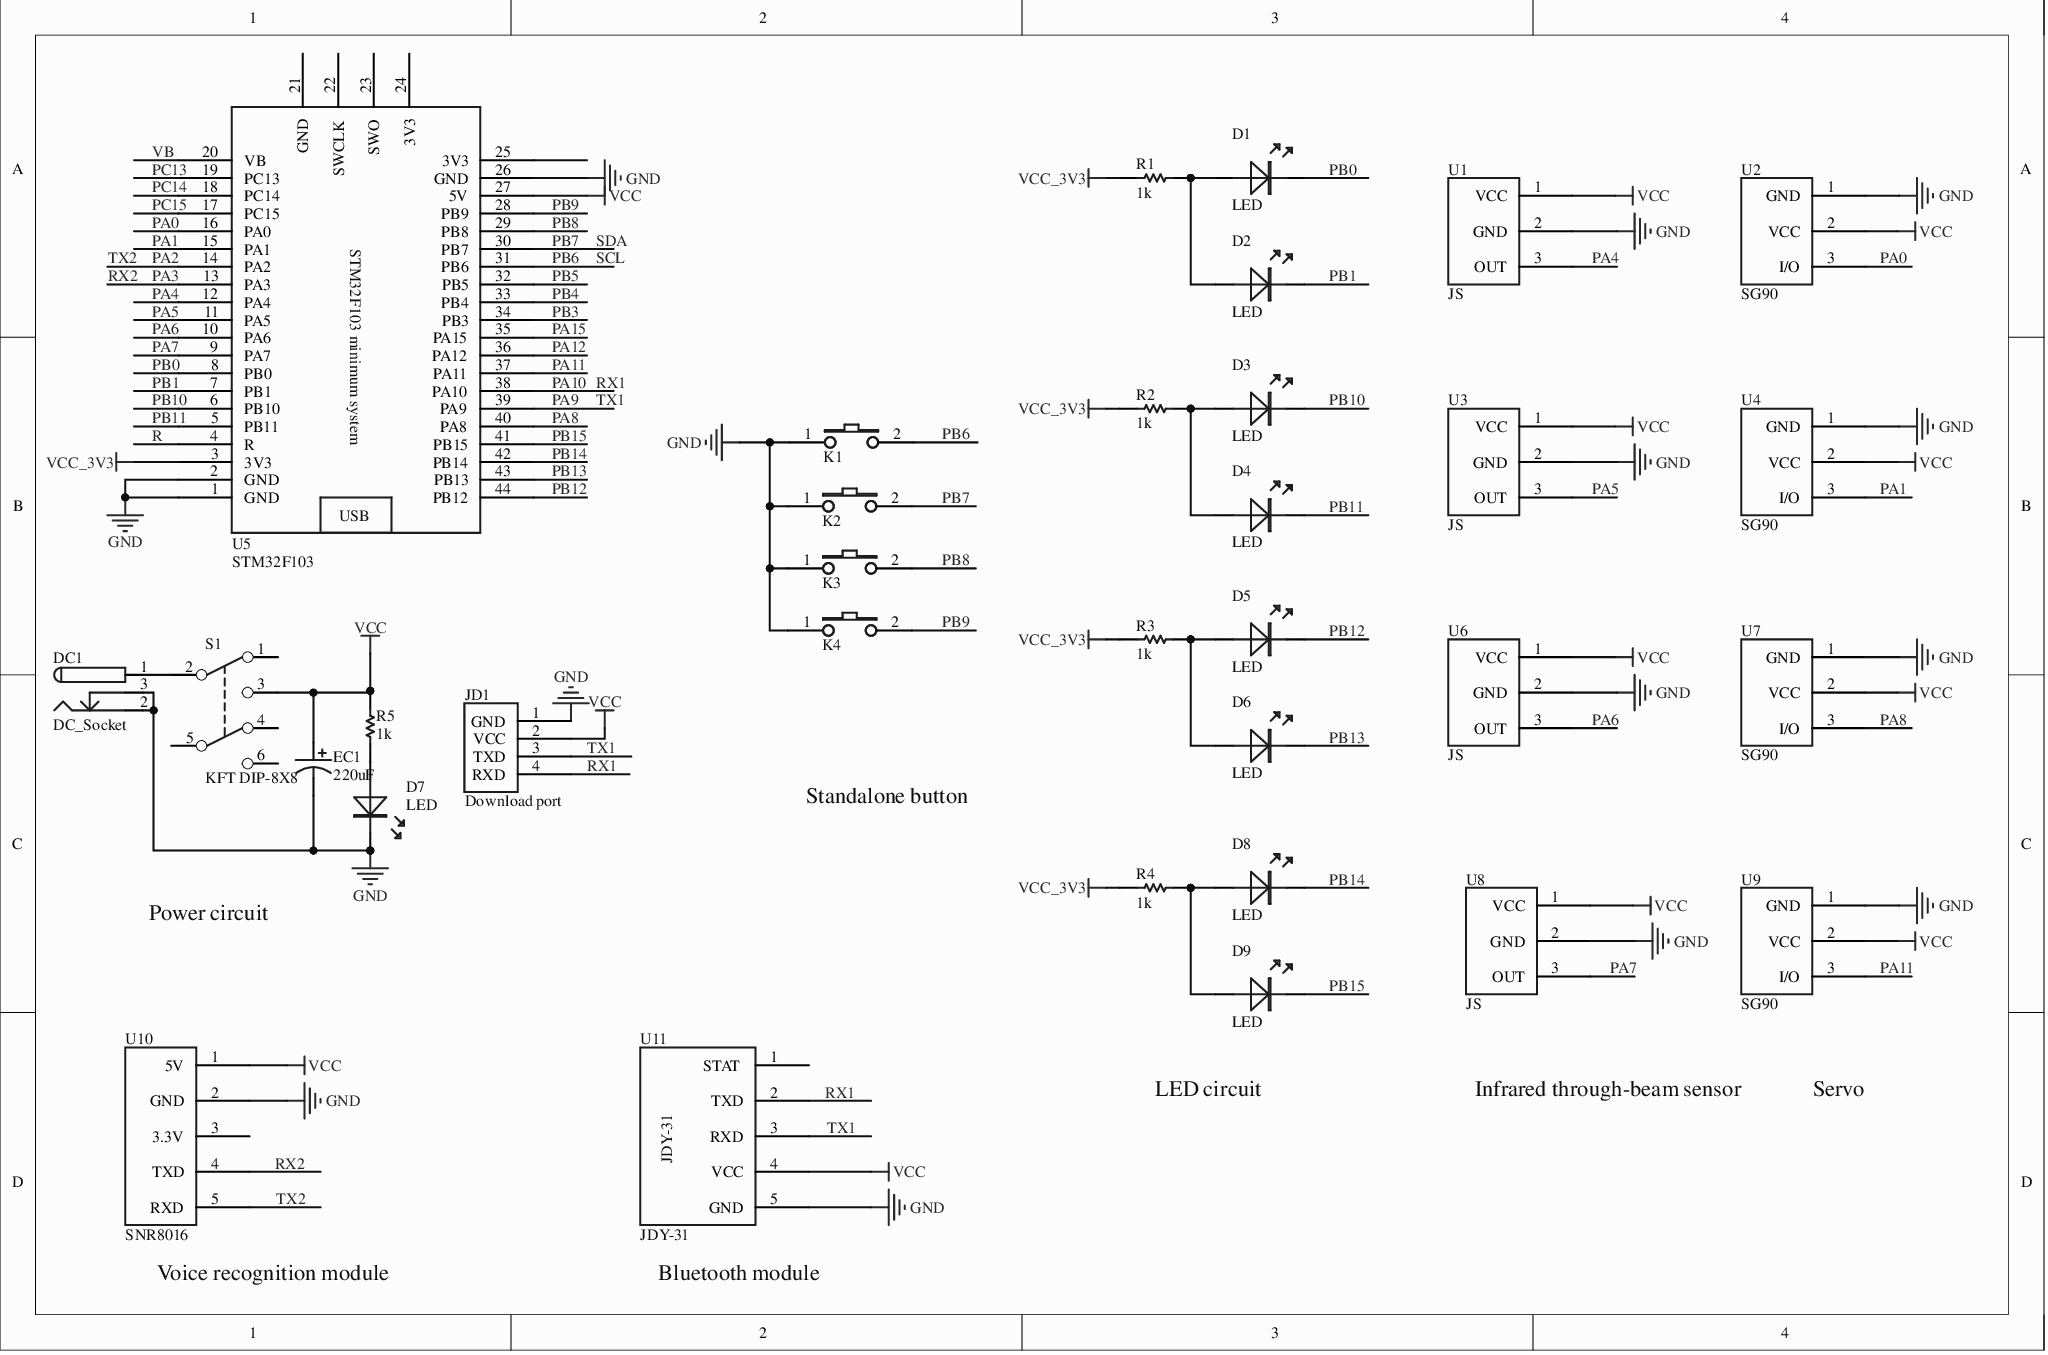
[diagram p0: MISC49929-2.schdoc]
# Altium project MISC49929.PrjPcb
1 sheet, 33 parts. Net scope: global (net labels, ports and power ports of the same name join across sheets).
Board file: MISC49929.pcbdoc

## Sheet MISC49929-2.schdoc
size 292 x 193 mm; Name: MISC49929

### Parts
D1  LED  [LED5-GRE]
D2  LED  [LED5-RED]
D3  LED  [LED5-GRE]
D4  LED  [LED5-RED]
D5  LED  [LED5-GRE]
D6  LED  [LED5-RED]
D7  LED  [LED5-GRE]
D8  LED  [LED5-GRE]
D9  LED  [LED5-RED]
DC1  DC_Socket  [DC-005]
EC1  220uF  [DIP-EC3.5X8X11.5]
JD1  Download port  [下载口]
K1  BUTTOM  [DIP-6X6X5]  (value not drawn)
K2  BUTTOM  [DIP-6X6X5]  (value not drawn)
K3  BUTTOM  [DIP-6X6X5]  (value not drawn)
K4  BUTTOM  [DIP-6X6X5]  (value not drawn)
R1  1k  [AXIAL0.3-1k]
R2  1k  [AXIAL0.3-1k]
R3  1k  [AXIAL0.3-1k]
R4  1k  [AXIAL0.3-1k]
R5  1k  [AXIAL0.3-1k]
S1  KFT DIP-8X8  [KFT DIP-8X8]
U1  JS  [JS]
U2  SG90  [SG90]
U3  JS  [JS]
U4  SG90  [SG90]
U5  STM32F103  [STM32F103]
U6  JS  [JS]
U7  SG90  [SG90]
U8  JS  [JS]
U9  SG90  [SG90]
U10  SNR8016  [SNR8016]
U11  JDY-31

### Nets
GND: D7.K DC1.2 DC1.3 EC1.2 JD1.1(GND) K1.1 K2.1 K3.1 K4.1 U1.2(GND) U2.1(GND) U3.2(GND) U4.1(GND) U5.1(GND) U5.2(GND) U5.26(GND) U6.2(GND) U7.1(GND) U8.2(GND) U9.1(GND) U10.2(GND) U11.5(GND)
VCC: EC1.1 JD1.2(VCC) R5.2 S1.3 U1.1(VCC) U2.2(VCC) U3.1(VCC) U4.2(VCC) U5.27(5V) U6.1(VCC) U7.2(VCC) U8.1(VCC) U9.2(VCC) U10.1(5V) U11.4(VCC)
VCC_3V3: R1.2 R2.2 R3.2 R4.2 U5.3(3V3)
PA0: U2.3(I/O) U5.16(PA0)
PA1: U4.3(I/O) U5.15(PA1)
PA2: U5.14(PA2) U10.5(RXD)  [also labelled TX2]
PA3: U5.13(PA3) U10.4(TXD)  [also labelled RX2]
PA4: U1.3(OUT) U5.12(PA4)
PA5: U3.3(OUT) U5.11(PA5)
PA6: U5.10(PA6) U6.3(OUT)
PA7: U5.9(PA7) U8.3(OUT)
PA8: U5.40(PA8) U7.3(I/O)
PA9: JD1.3(TXD) U5.39(PA9) U11.3(RXD)  [also labelled TX1]
PA10: JD1.4(RXD) U5.38(PA10) U11.2(TXD)  [also labelled RX1]
PA11: U5.37(PA11) U9.3(I/O)
PA12: U5.36(PA12)
PA15: U5.35(PA15)
PB0: D1.K U5.8(PB0)
PB1: D2.K U5.7(PB1)
PB3: U5.34(PB3)
PB4: U5.33(PB4)
PB5: U5.32(PB5)
PB6: K1.2 U5.31(PB6)  [also labelled SCL]
PB7: K2.2 U5.30(PB7)  [also labelled SDA]
PB8: K3.2 U5.29(PB8)
PB9: K4.2 U5.28(PB9)
PB10: D3.K U5.6(PB10)
PB11: D4.K U5.5(PB11)
PB12: D5.K U5.44(PB12)
PB13: D6.K U5.43(PB13)
PB14: D8.K U5.42(PB14)
PB15: D9.K U5.41(PB15)
PC13: U5.19(PC13)
PC14: U5.18(PC14)
PC15: U5.17(PC15)
R: U5.4(R)
VB: U5.20(VB)
NetD1_A: D1.A D2.A R1.1
NetD3_A: D3.A D4.A R2.1
NetD5_A: D5.A D6.A R3.1
NetD7_A: D7.A R5.1
NetD8_A: D8.A D9.A R4.1
NetDC1_1: DC1.1 S1.2

Not connected (* = marked no-connect by the designer): S1 1 4 5 6; U5 21(GND) 22(SWCLK) 23(SWO) 24(3V3) 25(3V3); U10 3(3.3V)*; U11 1(STAT)*

### Notes on the sheet
- Standalone button
- Power circuit
- LED circuit
- Infrared through-beam sensor
- Servo
- (near U10) Voice recognition module
- (near U11) Bluetooth module

### Library data of the parts
D1 = LED: LED red; Origin Footprint: LED5-BLUE; OriginFootprint 3: LED5-YEL; UniqueId: 07a0d5848cd81316; AddInBom: yes; Device: LED; OriginFootprint 2: LED5-GRE; DesignItemID: LED; LibraryName: LED; SymbolName: LED; FootprintName: LED5-GRE
D2 = LED_1: LED red; Origin Footprint: LED5-BLUE; OriginFootprint 2: LED5-GRE; OriginFootprint 3: LED5-YEL; UniqueId: fa5cd661465da5bc; AddInBom: yes; Device: LED_1; DesignItemID: LED; LibraryName: LED; SymbolName: LED; FootprintName: LED5-RED
D3 = LED: LED red; Origin Footprint: LED5-BLUE; OriginFootprint 3: LED5-YEL; UniqueId: ce0e29427420bb9a; AddInBom: yes; Device: LED; OriginFootprint 2: LED5-GRE; DesignItemID: LED; LibraryName: LED; SymbolName: LED; FootprintName: LED5-GRE
D4 = LED_1: LED red; Origin Footprint: LED5-BLUE; OriginFootprint 2: LED5-GRE; OriginFootprint 3: LED5-YEL; UniqueId: 671e3575a93d22ee; AddInBom: yes; Device: LED_1; DesignItemID: LED; LibraryName: LED; SymbolName: LED; FootprintName: LED5-RED
D5 = LED: LED red; Origin Footprint: LED5-BLUE; OriginFootprint 3: LED5-YEL; UniqueId: f6a2299b727f22e5; AddInBom: yes; Device: LED; OriginFootprint 2: LED5-GRE; DesignItemID: LED; LibraryName: LED; SymbolName: LED; FootprintName: LED5-GRE
D6 = LED_1: LED red; Origin Footprint: LED5-BLUE; OriginFootprint 2: LED5-GRE; OriginFootprint 3: LED5-YEL; UniqueId: da39aa9ccad1dedd; AddInBom: yes; Device: LED_1; DesignItemID: LED; LibraryName: LED; SymbolName: LED; FootprintName: LED5-RED
D7 = LED: LED green; Origin Footprint: LED5-BLUE; OriginFootprint 2: LED5-RED; OriginFootprint 3: LED5-YEL; UniqueId: cc99b6ab75b61af5; AddInBom: yes; Device: LED; DesignItemID: LED; LibraryName: LED; SymbolName: LED; FootprintName: LED5-GRE
D8 = LED: LED red; Origin Footprint: LED5-BLUE; OriginFootprint 3: LED5-YEL; UniqueId: fa1f7fcf59ad3572; AddInBom: yes; Device: LED; OriginFootprint 2: LED5-GRE; DesignItemID: LED; LibraryName: LED; SymbolName: LED; FootprintName: LED5-GRE
D9 = LED_1: LED red; Origin Footprint: LED5-BLUE; OriginFootprint 2: LED5-GRE; OriginFootprint 3: LED5-YEL; UniqueId: 24b3e8ded7e5fe7b; AddInBom: yes; Device: LED_1; DesignItemID: LED; LibraryName: LED; SymbolName: LED; FootprintName: LED5-RED
DC1 = DC_Socket: Power socket; UniqueId: 918354ff671956d3; AddInBom: yes; ModelId: bc01fa3fdb994156aa7bd7788425d33b; Device: DC_Socket; DesignItemID: DC_Socket; LibraryName: Power socket; SymbolName: DC_Socket; FootprintName: DC-005; ModelName: DC-005
EC1 = 220uF: Through-hole electrolytic capacitor; UniqueId: 1f6a804da79fa676; SymbolName: DIP_ECAP; AddInBom: yes; Device: 220uF; DesignItemID: DIP_ECAP; LibraryName: Electrolytic capacitor--220uF; FootprintName: DIP-EC3.5X8X11.5
JD1 = 下载口_1: Device: Download port_1; UniqueId: 8d67e1bcb20313ce; AddInBom: yes; DesignItemID: 下载口; LibraryName: Download port; Description: Download port; SymbolName: Download port; FootprintName: Download port
K1 = BUTTOM: Button; UniqueId: 28855386baaab8ba; AddInBom: yes; Device: BUTTOM; DesignItemID: BUTTOM; LibraryName: Reference; SymbolName: BUTTOM; FootprintName: DIP-6X6X5
K2 = BUTTOM: Button; UniqueId: e2dee5ee6a5fdee0; AddInBom: yes; Device: BUTTOM; DesignItemID: BUTTOM; LibraryName: Reference; SymbolName: BUTTOM; FootprintName: DIP-6X6X5
K3 = BUTTOM: Button; UniqueId: 177bbada0502c5f7; AddInBom: yes; Device: BUTTOM; DesignItemID: BUTTOM; LibraryName: Reference; SymbolName: BUTTOM; FootprintName: DIP-6X6X5
K4 = BUTTOM: Button; UniqueId: 787baf109c0c5026; AddInBom: yes; Device: BUTTOM; DesignItemID: BUTTOM; LibraryName: Reference; SymbolName: BUTTOM; FootprintName: DIP-6X6X5
R1 = 1k: Resistor; Origin Footprint: AXIAL0.3-3.3k; OriginFootprint 2: AXIAL0.3-10k; UniqueId: 4e166b190d4de1c3; SymbolName: RES; AddInBom: yes; Device: 1k; DesignItemID: RES; LibraryName: Resistor; FootprintName: AXIAL0.3-1k
R2 = 1k: Resistor; Origin Footprint: AXIAL0.3-3.3k; OriginFootprint 2: AXIAL0.3-10k; UniqueId: 06442d24ab060343; SymbolName: RES; AddInBom: yes; Device: 1k; DesignItemID: RES; LibraryName: Resistor; FootprintName: AXIAL0.3-1k
R3 = 1k: Resistor; Origin Footprint: AXIAL0.3-3.3k; OriginFootprint 2: AXIAL0.3-10k; UniqueId: 6e26aea592918673; SymbolName: RES; AddInBom: yes; Device: 1k; DesignItemID: RES; LibraryName: Resistor; FootprintName: AXIAL0.3-1k
R4 = 1k: Resistor; Origin Footprint: AXIAL0.3-3.3k; OriginFootprint 2: AXIAL0.3-10k; UniqueId: 49359f7360e76581; SymbolName: RES; AddInBom: yes; Device: 1k; DesignItemID: RES; LibraryName: Resistor; FootprintName: AXIAL0.3-1k
R5 = 1k: Resistor; Origin Footprint: AXIAL0.3-3.3k; OriginFootprint 2: AXIAL0.3-10k; UniqueId: 96bd3269827a783e; SymbolName: RES; AddInBom: yes; Device: 1k; DesignItemID: RES; LibraryName: Resistor; FootprintName: AXIAL0.3-1k
S1 = KFT DIP-8X8_1: Self-locking button; UniqueId: da892dff24010eb4; AddInBom: yes; Device: KFT DIP-8X8_1; DesignItemID: KFT DIP-8X8; LibraryName: Self-locking button; SymbolName: KFT DIP-8X8; FootprintName: KFT DIP-8X8
U1 = JS_2: Infrared through-beam sensor--counting; UniqueId: 48a4a086d8c42a18; AddInBom: yes; Device: JS_2; DesignItemID: JS; LibraryName: Infrared through-beam sensor-counting; SymbolName: JS; FootprintName: JS
U2 = SG90_1: Servo; UniqueId: d74c11912b695046; AddInBom: yes; Device: SG90_1; DesignItemID: SG90; LibraryName: Servo; SymbolName: SG90; FootprintName: SG90
U3 = JS_2: Infrared through-beam sensor--counting; UniqueId: eac3f191c372887e; AddInBom: yes; Device: JS_2; DesignItemID: JS; LibraryName: Infrared through-beam sensor-counting; SymbolName: JS; FootprintName: JS
U4 = SG90_1: Servo; UniqueId: e5d1bee62801ccc5; AddInBom: yes; Device: SG90_1; DesignItemID: SG90; LibraryName: Servo; SymbolName: SG90; FootprintName: SG90
U5 = STM32F103_1: UniqueId: 65fd737caad1a168; AddInBom: yes; Device: STM32F103_1; DesignItemID: STM32F103; LibraryName: Custom schematic library; Description: STM32F103; SymbolName: STM32F103; FootprintName: STM32F103
U6 = JS_2: Infrared through-beam sensor--counting; UniqueId: cb0a5e759a2bc85d; AddInBom: yes; Device: JS_2; DesignItemID: JS; LibraryName: Infrared through-beam sensor-counting; SymbolName: JS; FootprintName: JS
U7 = SG90_1: Servo; UniqueId: 917392894f3a2a5c; AddInBom: yes; Device: SG90_1; DesignItemID: SG90; LibraryName: Servo; SymbolName: SG90; FootprintName: SG90
U8 = JS_2: Infrared through-beam sensor--counting; UniqueId: 379bb34d70e5da90; AddInBom: yes; Device: JS_2; DesignItemID: JS; LibraryName: Infrared through-beam sensor-counting; SymbolName: JS; FootprintName: JS
U9 = SG90_1: Servo; UniqueId: 0cf0c6d72374702e; AddInBom: yes; Device: SG90_1; DesignItemID: SG90; LibraryName: Servo; SymbolName: SG90; FootprintName: SG90
U10 = SNR8016_1: Voice recognition module; UniqueId: 5152fb4fa8412479; AddInBom: yes; Device: SNR8016_1; DesignItemID: SNR8016; LibraryName: Voice recognition; SymbolName: SNR8016; FootprintName: SNR8016
U11 = JDY-31: Bluetooth; UniqueId: 8cd974130b34484c; AddInBom: yes; Device: JDY-31; Origin Footprint: JDY-31; DesignItemID: JDY-31; LibraryName: Bluetooth--JDY-31; SymbolName: JDY-31